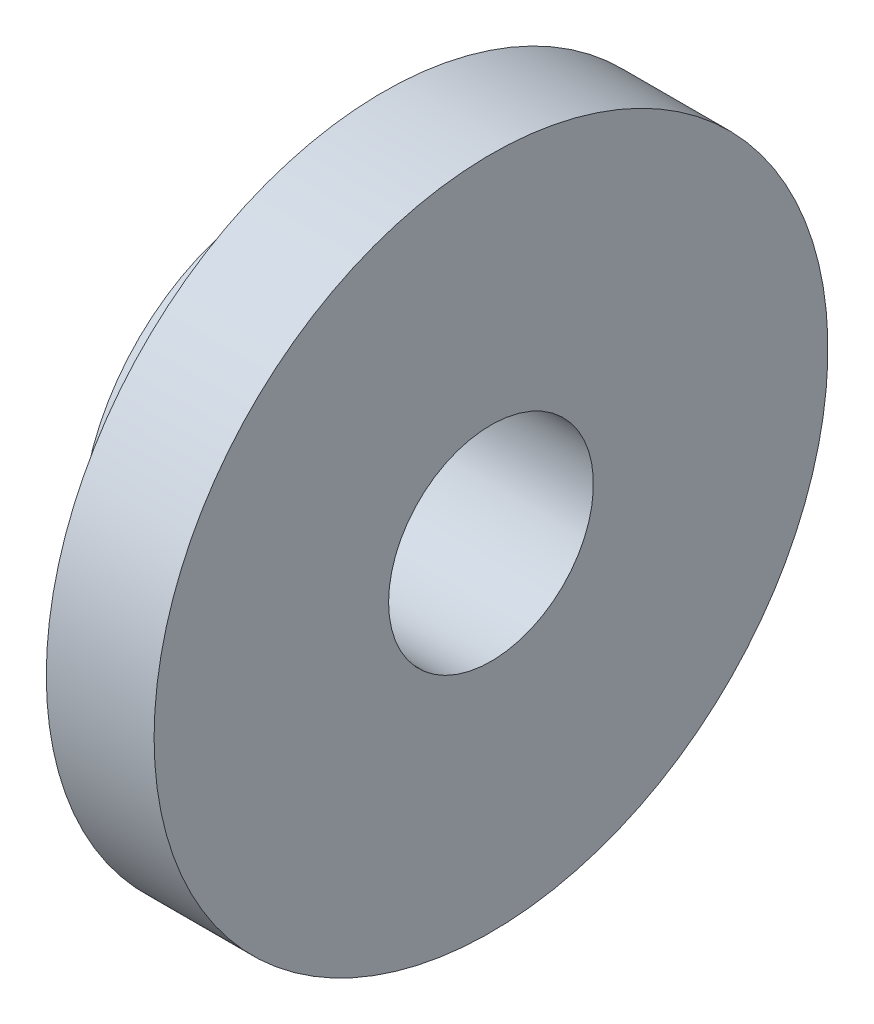
from build123d import *


with BuildPart() as part:
    # Sketch1 → Revolve1 (revolve)
    with BuildSketch(Plane.XY, mode=Mode.PRIVATE) as revolve1_sk:
        Polygon((0, -19), (0, -36), (20, -36), (20, -62.5), (40, -62.5), (40, -19), align=None)
    revolve(revolve1_sk.sketch.rotate(Axis((0, 0, 0), (1, 0, 0)), 270), axis=Axis((0, 0, 0), (1, 0, 0)))


solid = part.part
